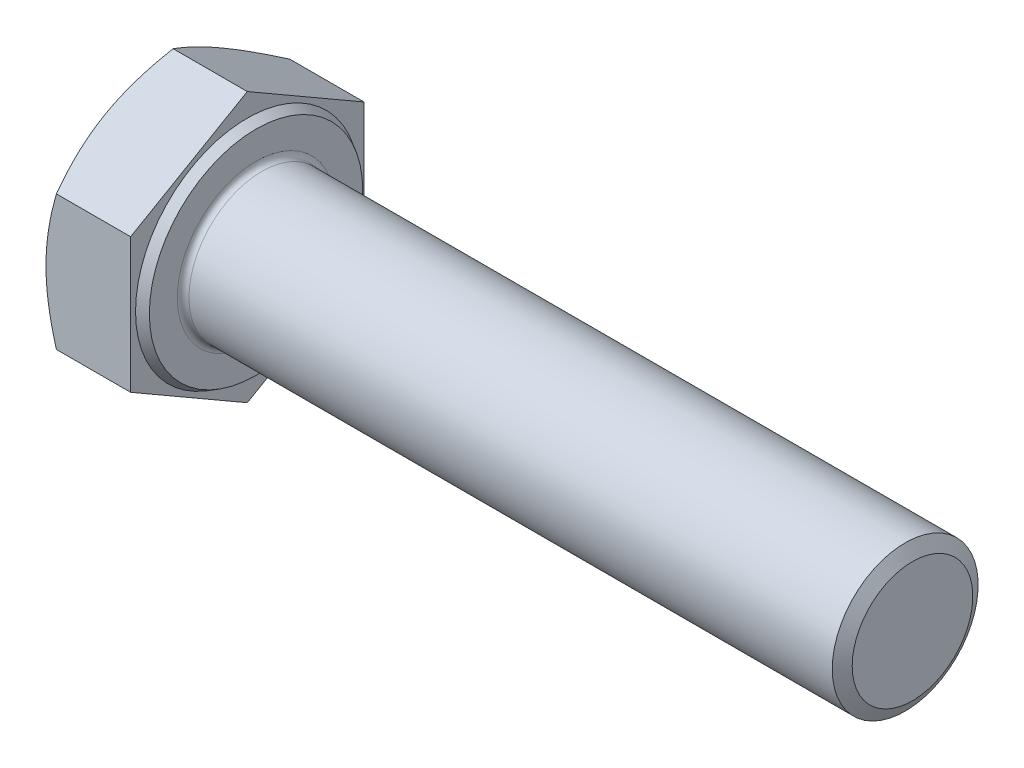
from build123d import *

# Parameters (mm, degrees)
EXTRUDE_419_DEPTH = 6.4
FILLET_1345_R     = 0.4


with BuildPart() as part:
    # 草图1 → Extrude 419 (new body)
    with BuildSketch(Plane(origin=(0, 0, 0), x_dir=(0, 0, -1), z_dir=(1, 0, 0))):
        Polygon((8, 4.618802154), (8, -4.618802154), (0, -9.237604307), (-8, -4.618802154), (-8, 4.618802154), (0, 9.237604307), align=None)
    extrude(amount=EXTRUDE_419_DEPTH)

    # 草图2 → 凸台-旋转1 (revolve)
    with BuildSketch(Plane.XY, mode=Mode.PRIVATE) as revolve_1_sk:
        Polygon((0, 0), (51.4, 0), (51.4, 4.134), (51.4, 5), (25.7, 5), (0, 5), align=None)
    revolve(revolve_1_sk.sketch.rotate(Axis((0, 0, 0), (1, 0, 0)), 90), axis=Axis((0, 0, 0), (1, 0, 0)))

    # 草图3 → 切除-旋转1 (revolve, cut)
    with BuildSketch(Plane.XY):
        Polygon((0, 8), (3.601282526, 14.237604307), (3.601282526, 19.237604307), (-10, 19.237604307), (-10, 8), align=None)
    revolve(axis=Axis((0, 0, 0), (1, 0, 0)), mode=Mode.SUBTRACT)

    # 草图4 → 切除-旋转3 (revolve, cut)
    with BuildSketch(Plane.XY, mode=Mode.PRIVATE) as cut_revolve_3_sk:
        Polygon((6.4, 7.315), (5.8, 7.661410162), (5.8, 9.237604307), (6.4, 9.237604307), align=None)
    revolve(cut_revolve_3_sk.sketch.rotate(Axis((0, 0, 0), (1, 0, 0)), 90), axis=Axis((0, 0, 0), (1, 0, 0)), mode=Mode.SUBTRACT)

    # Fillet 1345
    fillet_1345_edges = [part.edges().sort_by_distance(p)[0] for p in [
        (6.4, 0, -5),
    ]]
    fillet(fillet_1345_edges, radius=FILLET_1345_R)

    # 草图6 → 切除-旋转4 (revolve, cut)
    with BuildSketch(Plane.XY, mode=Mode.PRIVATE) as cut_revolve_4_sk:
        Polygon((50.9, 5), (51.9, 5), (51.4, 4.133974596), align=None)
    revolve(cut_revolve_4_sk.sketch.rotate(Axis((0, 0, 0), (1, 0, 0)), 90), axis=Axis((0, 0, 0), (1, 0, 0)), mode=Mode.SUBTRACT)


solid = part.part
